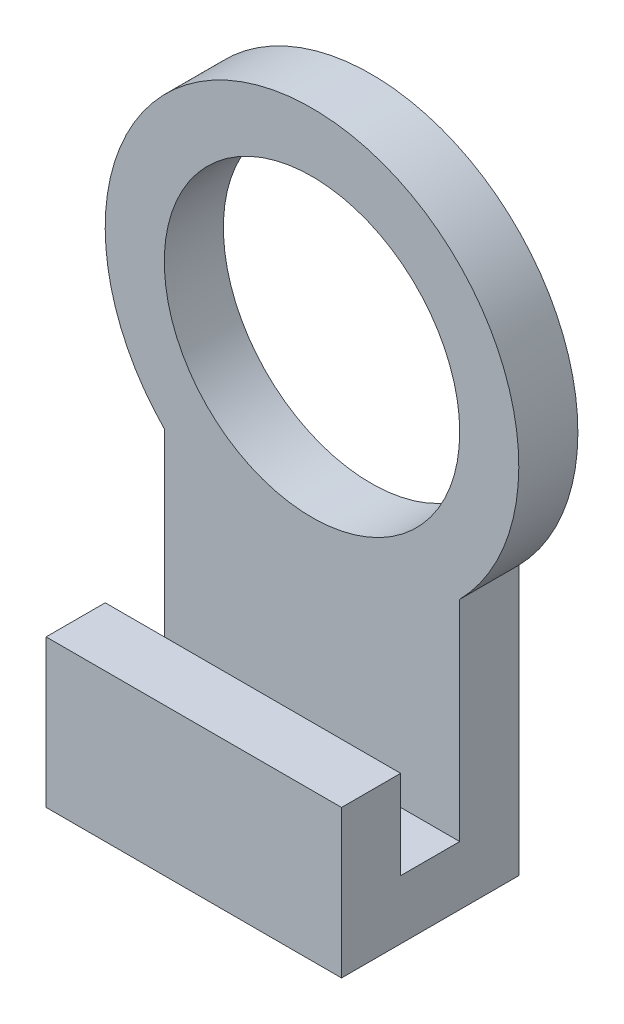
SolidWorks part; units mm, degrees
ref_plane "Front Plane" through (0, 0, 0) normal (0, 0, 1) x (1, 0, 0)
ref_plane "Top Plane" through (0, 0, 0) normal (0, 1, 0) x (1, 0, 0)
ref_plane "Right Plane" through (0, 0, 0) normal (1, 0, 0) x (0, 0, -1)
ref_plane "Plane1" through (0, 0, 0) normal (0, 0, -1) x (-1, 0, 0)
sketch "Sketch1" plane through (0, 0, 0) normal (0, 0, -1) x (-1, 0, 0)
  line L0 (-10, -28) -> (10, -28)
  line L1 (10, -28) -> (10, -9.798)
  line L2 (-10, -9.798) -> (-10, -28)
  arc A0 (10, -9.798) -> (-10, -9.798) centre (0, 0) ccw
extrude "Boss-Extrude1" add sketch "Sketch1" against normal blind 4
sketch "Sketch2" plane through (0, 0, 4) normal (0, 0, 1) x (1, 0, 0)
  line L0 (10, -24) -> (10, -28)
  line L1 (10, -28) -> (-10, -28)
  line L2 (-10, -28) -> (-10, -24)
  line L3 (-10, -24) -> (10, -24)
extrude "Boss-Extrude2" add sketch "Sketch2" along normal blind 8
sketch "Sketch3" plane through (0, -24, 0) normal (0, 1, 0) x (-1, 0, 0)
  line L0 (-10, 8) -> (-10, 12)
  line L1 (-10, 12) -> (10, 12)
  line L2 (10, 12) -> (10, 8)
  line L3 (10, 8) -> (-10, 8)
extrude "Boss-Extrude3" add sketch "Sketch3" along normal blind 6
hole_wizard "Ø20.0 (20) Diameter Hole1" positions "Sketch5" profile "Sketch4" hole size "Ø20.0" standard "ANSI Metric"
sketch "Sketch5" plane through (0, 0, 4) normal (0, 0, 1) x (1, 0, 0)
  point P0 (0, 0)
sketch "Sketch4" plane through (0, 0, 4) normal (1, 0, 0) x (0, -1, 0)
  line L0 (0, 0) -> (0, 4)
  line L1 (0, 4) -> (10, 4)
  line L2 (10, 4) -> (10, 0)
  line L5 (10, 0) -> (0, 0)
  line L11 (0, -6.35) -> (0, 107.95) construction
  dimension "通孔孔直径" = 20
  dimension "通孔孔深度" = 4
